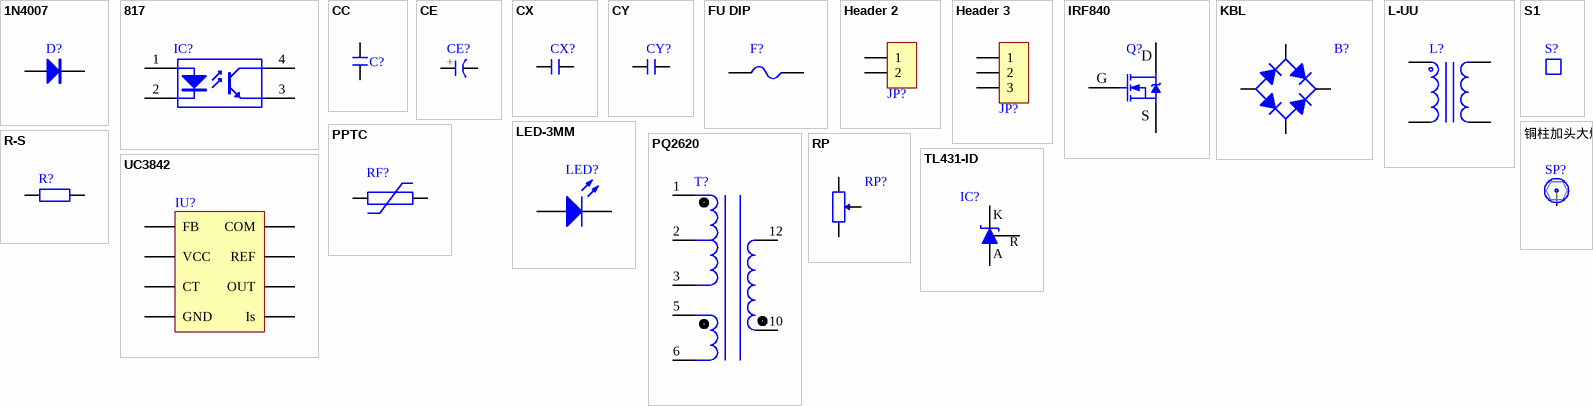
[diagram p0: symbols 1N4007 to 铜柱加头大焊盘]
# Altium schematic symbol library MISC82119-2.SCHLIB: 21 symbols
Pins are listed as number, name and electrical type; pins without a type are passive.


## 1N4007
designator D?
Rectifier diode
footprint TO220A (220, 3-pin transistor.)
footprint SOD-123 (2.7x1.6x1.1mm (L*W*H, excluding leads))
footprint SMA (4.5x2.6*2.2mm (L*W*H, excluding leads))
footprint DO-41V (2.6*3.5mm (diameter, pin pitch))
pins: 1 A, 2 K

## 817
designator IC?
Linear optocoupler
footprint DIP4-300 (4.6*7.6*3.8 (L*W*H))
pins: 1 A "Anode", 2 K "Cathode", 3 E "Emitter", 4 C "Collector"

## CC
designator C?
Ceramic disc capacitor
footprint CC 1.8*3.6 (Pin pitch 1.8mm, diameter 3.6mm)
footprint CC 2.2*5 (Pin pitch 2.2mm, diameter 5mm)
footprint CY 5*7*2.5
pins: 1, 2

## CE
designator CE?
Through-hole electrolytic capacitor
footprint CAP 1.5*4*8 (Pin pitch 1.5mm, diameter 4mm, height 8mm)
footprint CAP 1.5*4*8 - BK (Pin pitch 1.5mm, diameter 4mm, height 8mm)
footprint CAP 1.5*4*8 - GD (Pin pitch 1.5mm, diameter 4mm, height 8mm)
footprint CAP 1.5*4*8-H (Pin pitch 1.5mm, diameter 4mm, height 8mm)
footprint CAP 1.5*4*8-H - BK (Pin pitch 1.5mm, diameter 4mm, height 8mm)
footprint CAP 1.5*4*8-H - GD (Pin pitch 1.5mm, diameter 4mm, height 8mm)
footprint CAP 2.0*5*11 (Pin pitch 2mm, diameter 5mm, height 11mm)
footprint CAP 2.0*5*11 - BK (Pin pitch 2mm, diameter 5mm, height 11mm)
footprint CAP 2.0*5*11 - GD (Pin pitch 2mm, diameter 5mm, height 11mm)
footprint CAP 2.0*5*11-H (Pin pitch 2mm, diameter 5mm, height 11mm)
footprint CAP 2.0*5*11-H - BK (Pin pitch 2mm, diameter 5mm, height 11mm)
footprint CAP 2.0*5*11-H - GD (Pin pitch 2mm, diameter 5mm, height 11mm)
footprint CAP 2.5*5*11 (Pin pitch 2.5mm, diameter 5mm, height 11mm)
footprint CAP 2.5*5*11 - BK (Pin pitch 2.5mm, diameter 5mm, height 11mm)
footprint CAP 2.5*5*11 - GD (Pin pitch 2.5mm, diameter 5mm, height 11mm)
footprint CAP 2.5*5*11-H (Pin pitch 2.5mm, diameter 5mm, height 11mm)
footprint CAP 2.5*5*11-H - BK (Pin pitch 2.5mm, diameter 5mm, height 11mm)
footprint CAP 2.5*5*11-H - GD (Pin pitch 2.5mm, diameter 5mm, height 11mm)
footprint CAP 2.5*6.3*7 (Pin pitch 2.5mm, diameter 6.3mm, height 7mm)
footprint CAP 2.5*6.3*7 - BK (Pin pitch 2.5mm, diameter 6.3mm, height 7mm)
footprint CAP 2.5*6.3*7 - GD (Pin pitch 2.5mm, diameter 6.3mm, height 7mm)
footprint CAP 2.5*6.3*7-H (Pin pitch 2.5mm, diameter 6.3mm, height 7mm)
footprint CAP 2.5*6.3*7-H - BK (Pin pitch 2.5mm, diameter 6.3mm, height 7mm)
footprint CAP 2.5*6.3*7-H - GD (Pin pitch 2.5mm, diameter 6.3mm, height 7mm)
footprint CAP 2.5*6.3*11.2 (Pin pitch 2.5mm, diameter 6.3mm, height 11.2mm)
footprint CAP 2.5*6.3*11.2 - BK (Pin pitch 2.5mm, diameter 6.3mm, height 11.2mm)
footprint CAP 2.5*6.3*11.2 - GD (Pin pitch 2.5mm, diameter 6.3mm, height 11.2mm)
footprint CAP 2.5*6.3*11.2-H (Pin pitch 2.5mm, diameter 6.3mm, height 11.2mm)
footprint CAP 2.5*6.3*11.2-H - BK (Pin pitch 2.5mm, diameter 6.3mm, height 11.2mm)
footprint CAP 2.5*6.3*11.2-H - GD (Pin pitch 2.5mm, diameter 6.3mm, height 11.2mm)
footprint CAP 3.5*8*11.5 (Pin pitch 3.5mm, diameter 8mm, height 11.5mm)
footprint CAP 3.5*8*11.5 - BK (Pin pitch 3.5mm, diameter 8mm, height 11.5mm)
footprint CAP 3.5*8*11.5 - GD (Pin pitch 3.5mm, diameter 8mm, height 11.5mm)
footprint CAP 3.5*8*11.5-H (Pin pitch 3.5mm, diameter 8mm, height 11.5mm)
footprint CAP 3.5*8*11.5-H - BK (Pin pitch 3.5mm, diameter 8mm, height 11.5mm)
footprint CAP 3.5*8*11.5-H - GD (Pin pitch 3.5mm, diameter 8mm, height 11.5mm)
footprint CAP 5.0*10*12.5 (Pin pitch 5mm, diameter 10mm, height 12.5mm)
footprint CAP 5.0*10*12.5 - BK (Pin pitch 5mm, diameter 10mm, height 12.5mm)
footprint CAP 5.0*10*12.5 - GD (Pin pitch 5mm, diameter 10mm, height 12.5mm)
footprint CAP 5.0*10*12.5-H (Pin pitch 5mm, diameter 10mm, height 12.5mm)
footprint CAP 5.0*10*12.5-H - BK (Pin pitch 5mm, diameter 10mm, height 12.5mm)
footprint CAP 5.0*10*12.5-H - GD (Pin pitch 5mm, diameter 10mm, height 12.5mm)
footprint CAP 5.0*10*16 (Pin pitch 5mm, diameter 10mm, height 16mm)
footprint CAP 5.0*10*16 - BK (Pin pitch 5mm, diameter 10mm, height 16mm)
footprint CAP 5.0*10*16 - GD (Pin pitch 5mm, diameter 10mm, height 16mm)
footprint CAP 5.0*10*16-H (Pin pitch 5mm, diameter 10mm, height 16mm)
footprint CAP 5.0*10*16-H - BK (Pin pitch 5mm, diameter 10mm, height 16mm)
footprint CAP 5.0*10*16-H - GD (Pin pitch 5mm, diameter 10mm, height 16mm)
footprint CAP 5.0*10*20 (Pin pitch 5mm, diameter 10mm, height 20mm)
footprint CAP 5.0*10*20 - BK (Pin pitch 5mm, diameter 10mm, height 20mm)
footprint CAP 5.0*10*20 - GD (Pin pitch 5mm, diameter 10mm, height 20mm)
footprint CAP 5.0*10*20-H (Pin pitch 5mm, diameter 10mm, height 20mm)
footprint CAP 5.0*10*20-H - BK (Pin pitch 5mm, diameter 10mm, height 20mm)
footprint CAP 5.0*10*20-H - GD (Pin pitch 5mm, diameter 10mm, height 20mm)
footprint CAP 5.0*12.5*20 (Pin pitch 5mm, diameter 12.5mm, height 20mm)
footprint CAP 5.0*12.5*20 - BK (Pin pitch 5mm, diameter 12.5mm, height 20mm)
footprint CAP 5.0*12.5*20 - GD (Pin pitch 5mm, diameter 12.5mm, height 20mm)
footprint CAP 5.0*12.5*20-H (Pin pitch 5mm, diameter 12.5mm, height 20mm)
footprint CAP 5.0*12.5*20-H - BK (Pin pitch 5mm, diameter 12.5mm, height 20mm)
footprint CAP 5.0*12.5*20-H - GD (Pin pitch 5mm, diameter 12.5mm, height 20mm)
footprint CAP 5.0*12.5*25 (Pin pitch 5mm, diameter 12.5mm, height 25mm)
footprint CAP 5.0*12.5*25 - BK (Pin pitch 5mm, diameter 12.5mm, height 25mm)
footprint CAP 5.0*12.5*25 - GD (Pin pitch 5mm, diameter 12.5mm, height 25mm)
footprint CAP 5.0*12.5*25-H (Pin pitch 5mm, diameter 12.5mm, height 25mm)
footprint CAP 5.0*12.5*25-H - BK (Pin pitch 5mm, diameter 12.5mm, height 25mm)
footprint CAP 5.0*12.5*25-H - GD (Pin pitch 5mm, diameter 12.5mm, height 25mm)
footprint CAP 7.5*16*25 (Pin pitch 7.5mm, diameter 16mm, height 25mm)
footprint CAP 7.5*16*25 - BK (Pin pitch 7.5mm, diameter 16mm, height 25mm)
footprint CAP 7.5*16*25 - GD (Pin pitch 7.5mm, diameter 16mm, height 25mm)
footprint CAP 7.5*16*25-H (Pin pitch 7.5mm, diameter 16mm, height 25mm)
footprint CAP 7.5*16*25-H - BK (Pin pitch 7.5mm, diameter 16mm, height 25mm)
footprint CAP 7.5*16*25-H - GD (Pin pitch 7.5mm, diameter 16mm, height 25mm)
footprint CAP 7.5*16*31.5 (Pin pitch 7.5mm, diameter 16mm, height 31.5mm)
footprint CAP 7.5*16*31.5 - BK (Pin pitch 7.5mm, diameter 16mm, height 31.5mm)
footprint CAP 7.5*16*31.5 - GD (Pin pitch 7.5mm, diameter 16mm, height 31.5mm)
footprint CAP 7.5*16*31.5-H (Pin pitch 7.5mm, diameter 16mm, height 31.5mm)
footprint CAP 7.5*16*31.5-H - BK (Pin pitch 7.5mm, diameter 16mm, height 31.5mm)
footprint CAP 7.5*16*31.5-H - GD (Pin pitch 7.5mm, diameter 16mm, height 31.5mm)
footprint CAP 7.5*18*35.5 (Pin pitch 7.5mm, diameter 18mm, height 35.5mm)
footprint CAP 7.5*18*35.5 - BK (Pin pitch 7.5mm, diameter 18mm, height 35.5mm)
footprint CAP 7.5*18*35.5 - GD (Pin pitch 7.5mm, diameter 18mm, height 35.5mm)
footprint CAP 7.5*18*35.5-H (Pin pitch 7.5mm, diameter 18mm, height 35.5mm)
footprint CAP 7.5*18*35.5-H - BK (Pin pitch 7.5mm, diameter 18mm, height 35.5mm)
footprint CAP 7.5*18*35.5-H - GD (Pin pitch 7.5mm, diameter 18mm, height 35.5mm)
footprint CAP 10*22*31.5 (Pin pitch 10mm, diameter 22mm, height 31.5mm)
footprint CAP 10*22*31.5 - BK (Pin pitch 10mm, diameter 22mm, height 31.5mm)
footprint CAP 10*22*31.5 - GD (Pin pitch 10mm, diameter 22mm, height 31.5mm)
footprint CAP 10*22*40 (Pin pitch 10mm, diameter 22mm, height 40mm)
footprint CAP 10*22*40 - BK (Pin pitch 10mm, diameter 22mm, height 40mm)
footprint CAP 10*22*40 - GD (Pin pitch 10mm, diameter 22mm, height 40mm)
pins: 1 A, 2 K

## CX
designator CX?
Safety X capacitor
footprint CX 10-13*11
footprint CX 15*18*11 (Pin pitch 15mm, height 18mm, thickness 11mm)
pins: 1, 2

## CY
designator CY?
Safety Y capacitor
footprint CY 7.5*8*4 (Pin pitch 7.5mm, diameter 8mm, thickness 4mm)
footprint CY 7.5*10*4 (Pin pitch 7.5mm, diameter 10mm, thickness 4mm)
footprint CY 7.5*12*5 (Pin pitch 7.5mm, diameter 12mm, thickness 5mm)
footprint CY 10*14*5 (Pin pitch 10mm, diameter 14mm, thickness 5mm)
footprint CY 10*16*6 (Pin pitch 10mm, diameter 16mm, thickness 6mm)
footprint CY 10*18*6 (Pin pitch 10mm, diameter 18mm, thickness 6mm)
footprint CY 5*7*2.5 (Pin pitch 5mm, diameter 7mm, thickness 2.5mm)
pins: 1, 2

## FU DIP
designator F?
Through-hole fuse
footprint FU 4x16_V (4*16mm (diameter, pin pitch))
footprint FU 4x16_V (4*16mm (diameter, pin pitch))
pins: 1, 2

## Header 2
designator JP?
2P connector
footprint KF7620-2P (15.2*12*12mm (L*W*H))
pins: 1, 2

## Header 3
designator JP?
3P connector
footprint KF7620-3P (22.8*12*12mm (L*W*H))
pins: 1, 2, 3

## IRF840
designator Q?
N-channel MOSFET
footprint TO220A
footprint TO220A
footprint TO220C (220, 3-pin transistor)
pins: 1 G, 2 D, 3 S

## KBL
designator B?
600V/8A bridge rectifier
footprint KBL (19*6.25*15.7mm (L*W*H))
pins: AC1, AC2, DC+, DC-

## L-UU
designator L?
Common-mode choke
footprint UU9.8 (17*12*17mm (L*W*H))
footprint UU10.5 (18*16*20mm (L*W*H))
footprint UU16 (22*17.5*23mm (L*W*H))
footprint T12x6x4 (Diameter 13.2mm, thickness 7.2mm, pin pitch 5*6.6mm)
pins: 1, 2, 3, 4

## LED-3MM
designator LED?
Through-hole 3mm LED
footprint LED 3MM-B (Blue 3mm through-hole LED)
footprint LED 3MM-G (Green 3mm through-hole LED)
footprint LED 3MM-R (Red 3mm through-hole LED)
footprint LED 3MM-Y (Yellow 3mm through-hole LED)
footprint LED 3MM-YC (Orange 3mm through-hole LED)
footprint LED 3MM-W (White 3mm through-hole LED)
pins: 1 A, 2 K

## PPTC
designator RF?
PPTC resettable fuse
footprint TVR-10D
pins: 1, 2

## PQ2620
designator T?
12V high-frequency transformer
footprint PQ2625+6PIN (Footprint not found)
pins: 1, 2, 3, 5, 6, 10, 12

## R-S
designator R?
Color-band resistor
footprint RS 1/2W (Through-hole color-band resistor, pin pitch 12.5mm, diameter 3mm)
footprint RS 1/2W-V4 (Through-hole color-band resistor, pin pitch 4mm, diameter 3mm)
footprint RS 1/4W (Through-hole color-band resistor, pin pitch 9mm, diameter 2.3mm)
footprint RS 1/4W-V3 (Through-hole color-band resistor, pin pitch 3mm, diameter 2.3mm)
footprint RS 1/8W (Through-hole color-band resistor, pin pitch 6mm, diameter 1.5mm)
footprint RS 1/8W-V2 (Through-hole color-band resistor, pin pitch 2mm, diameter 1.5mm)
footprint RS 1W (Through-hole color-band resistor, pin pitch 15mm, diameter 4mm)
footprint RS 1W-F5 (Through-hole color-band resistor, pin pitch 15mm, diameter 4mm, standoff 5mm)
footprint RS 1W-V5 (Through-hole color-band resistor, pin pitch 5mm, diameter 4mm)
footprint RS 2W (Through-hole color-band resistor, pin pitch 20mm, diameter 5mm)
footprint RS 2W-F5 (Through-hole color-band resistor, pin pitch 20mm, diameter 5mm, standoff 5mm)
footprint RS 2W-V6 (Through-hole color-band resistor, pin pitch 6mm, diameter 5mm)
footprint RS 3W (Through-hole color-band resistor, pin pitch 25mm, diameter 6mm)
footprint RS 3W-F5 (Through-hole color-band resistor, pin pitch 25mm, diameter 6mm, standoff 5mm)
footprint RS 3W-V7 (Through-hole color-band resistor, pin pitch 7mm, diameter 6mm)
footprint RS 5W (Through-hole color-band resistor, pin pitch 30mm, diameter 8mm)
footprint RS 5W-F5 (Through-hole color-band resistor, pin pitch 30mm, diameter 8mm, standoff 5mm)
footprint RS 5W-V8 (Through-hole color-band resistor, pin pitch 8mm, diameter 8mm)
pins: 1, 2

## RP
designator RP?
Single-gang potentiometer
footprint 3296W (Precise Multi-Winding Adjustable Resistor)
footprint 3306W
footprint 3319P
footprint 3362P
footprint 3386W
footprint RM065 (Blue-white adjustable potentiometer)
footprint WH148-1-G15 (Single-gang potentiometer, pin pitch 5mm, shaft length 15mm)
footprint WH148-1-G18 (Single-gang potentiometer, pin pitch 5mm, shaft length 18mm)
footprint WH148-1-G20 (Single-gang potentiometer, pin pitch 5mm, shaft length 20mm)
footprint WH148-1-G25 (Single-gang potentiometer, pin pitch 5mm, shaft length 25mm)
footprint 3266W (L 7mm, W 4.8mm, H 7.5mm)
footprint 3266X (L 7mm, W 4.8mm, H 7.5mm)
footprint 3266Y (L 7mm, W 4.8mm, H 7.5mm)
footprint 3266Z (L 7mm, W 4.8mm, H 7.5mm)
footprint XV09223NPV-20F (L 9.85mm, W 11.55mm, H 20mm)
footprint XV09223NPV-25F (L 9.85mm, W 11.55mm, H 25mm)
footprint XV09223NPV-30F (L 9.85mm, W 11.55mm, H 30mm)
footprint 3006P (19.05mm*4.83mm*6.35mm (L*W*H))
pins: 1, 2, 3

## S1
designator S?
Heatsink
footprint SRP10-15-21 (10mm*15mm*21mm (L*W*H))
footprint SRP10-15-21-P (10mm*15mm*21mm (L*W*H))
footprint SRP10-15-21-W (10mm*15mm*21mm (L*W*H))
footprint SRP10-15-25 (10mm*15mm*25mm (L*W*H))
footprint SRP10-15-25-P (10mm*15mm*25mm (L*W*H))
footprint SRP10-15-25-W (10mm*15mm*25mm (L*W*H))
footprint SRP12-34-25-P (12mm*32mm*25mm (L*W*H))
footprint SRP16-24-25 (16mm*24mm*25mm (L*W*H))
footprint SRP16-24-25-P (16mm*24mm*25mm (L*W*H))
footprint SRP16-24-25-W (16mm*24mm*25mm (L*W*H))

## TL431-ID
designator IC?
Adjustable precision shunt regulator
footprint TO92A (92 transistor)
footprint TO92B (92 transistor)
pins: 1 R, 2 A, 3 K

## UC3842
designator IU?
footprint DIP8-300 (9.4*7.6*3.8 (L*W*H))
pins: 1 COM, 2 FB, 3 Is, 4 CT, 5 GND, 6 OUT, 7 VCC, 8 REF

## 铜柱加头大焊盘
designator SP?
Copper standoff
footprint M3x4+6_N (M3 standoff, length 4mm, thread length 6mm)
footprint M3x5+6_N (M3 standoff, length 5mm, thread length 6mm)
footprint M3x6+6_N (M3 standoff, length 6mm, thread length 6mm)
footprint M3x7+6_N (M3 standoff, length 7mm, thread length 6mm)
footprint M3x8+6_N (M3 standoff, length 8mm, thread length 6mm)
footprint M3x9+6_N (M3 standoff, length 9mm, thread length 6mm)
footprint M3x10+6_N (M3 standoff, length 10mm, thread length 6mm)
footprint M3x11+6_N (M3 standoff, length 11mm, thread length 6mm)
footprint M3x12+6_N (M3 standoff, length 12mm, thread length 6mm)
footprint M3x13+6_N (M3 standoff, length 13mm, thread length 6mm)
footprint M3x14+6_N (M3 standoff, length 14mm, thread length 6mm)
footprint M3x15+6_N (M3 standoff, length 15mm, thread length 6mm)
footprint M3x16+6_N (M3 standoff, length 16mm, thread length 6mm)
footprint M3x17+6_N (M3 standoff, length 17mm, thread length 6mm)
footprint M3x18+6_N (M3 standoff, length 18mm, thread length 6mm)
footprint M3x19+6_N (M3 standoff, length 19mm, thread length 6mm)
footprint M3x20+6_N (M3 standoff, length 20mm, thread length 6mm)
footprint M3x21+6_N (M3 standoff, length 21mm, thread length 6mm)
footprint M3x22+6_N (M3 standoff, length 22mm, thread length 6mm)
footprint M3x23+6_N (M3 standoff, length 23mm, thread length 6mm)
footprint M3x24+6_N (M3 standoff, length 24mm, thread length 6mm)
footprint M3x25+6_N (M3 standoff, length 25mm, thread length 6mm)
footprint M3x26+6_N (M3 standoff, length 26mm, thread length 6mm)
footprint M3x27+6_N (M3 standoff, length 27mm, thread length 6mm)
footprint M3x28+6_N (M3 standoff, length 28mm, thread length 6mm)
footprint M3x30+6_N (M3 standoff, length 30mm, thread length 6mm)
footprint M3x32+6_N (M3 standoff, length 32mm, thread length 6mm)
footprint M3x35+6_N (M3 standoff, length 35mm, thread length 6mm)
footprint M3x40+6_N (M3 standoff, length 40mm, thread length 6mm)
footprint M3x45+6_N (M3 standoff, length 45mm, thread length 6mm)
footprint M3x50+6_N (M3 standoff, length 50mm, thread length 6mm)
footprint M3x55+6_N (M3 standoff, length 55mm, thread length 6mm)
footprint M3x60+6_N (M3 standoff, length 60mm, thread length 6mm)
footprint M3x65+6_N (M3 standoff, length 65mm, thread length 6mm)
pins: 1